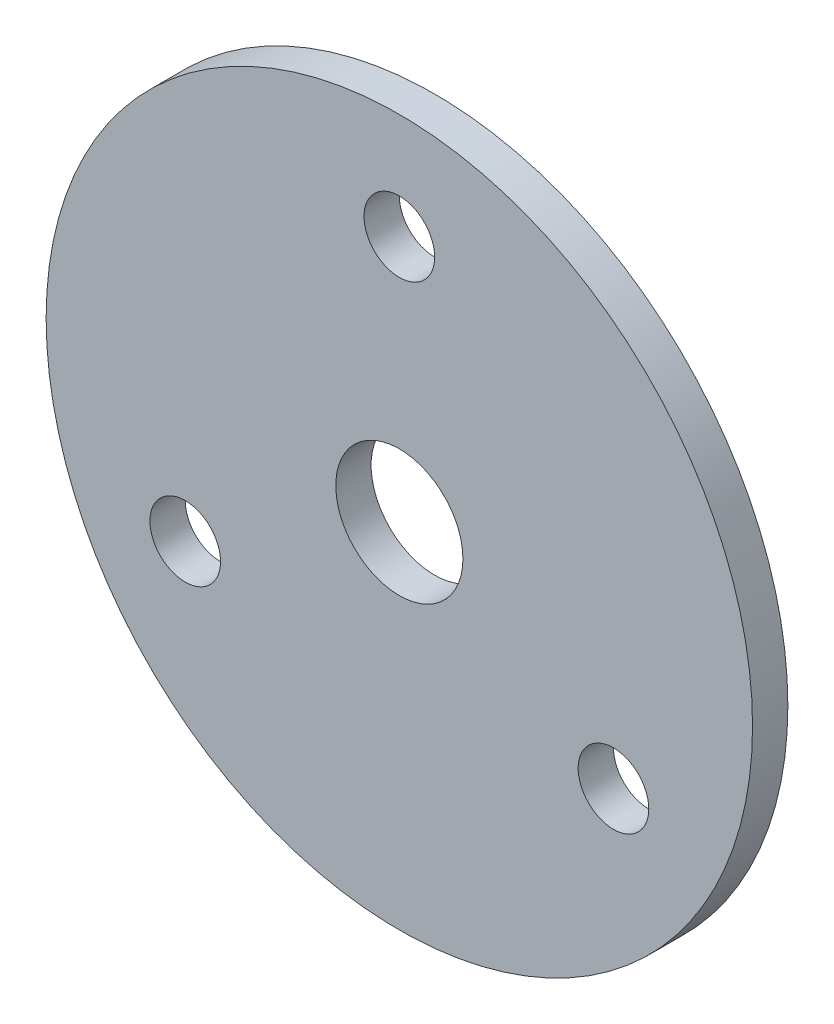
from build123d import *

# Parameters (mm, degrees)
SKETCH1_R           = 50
BOSS_EXTRUDE1_DEPTH = 5
SKETCH2_R           = 5
CUT_EXTRUDE1_DEPTH  = 5
CIRPATTERN1_COUNT   = 3
SKETCH3_R           = 9
CUT_EXTRUDE2_DEPTH  = 5


with BuildPart() as part:
    # Sketch1 → Boss-Extrude1 (new body)
    with BuildSketch(Plane.XY):
        Circle(SKETCH1_R)
    extrude(amount=BOSS_EXTRUDE1_DEPTH)

    # Sketch2 → Cut-Extrude1 (cut)
    with BuildSketch(Plane.XY.offset(5)):
        with Locations((0, 35)):
            Circle(SKETCH2_R)
    cut_extrude1 = extrude(amount=-CUT_EXTRUDE1_DEPTH, mode=Mode.SUBTRACT)

    # CirPattern1: Cut-Extrude1 ×3 about axis
    cirpattern1_axis = Axis((0, 0, 0), (0, 0, 1))
    for i in range(1, CIRPATTERN1_COUNT):
        add(cut_extrude1.rotate(cirpattern1_axis, i * 360 / CIRPATTERN1_COUNT), mode=Mode.SUBTRACT)

    # Sketch3 → Cut-Extrude2 (cut)
    with BuildSketch(Plane.XY.offset(5)):
        Circle(SKETCH3_R)
    extrude(amount=-CUT_EXTRUDE2_DEPTH, mode=Mode.SUBTRACT)


solid = part.part
